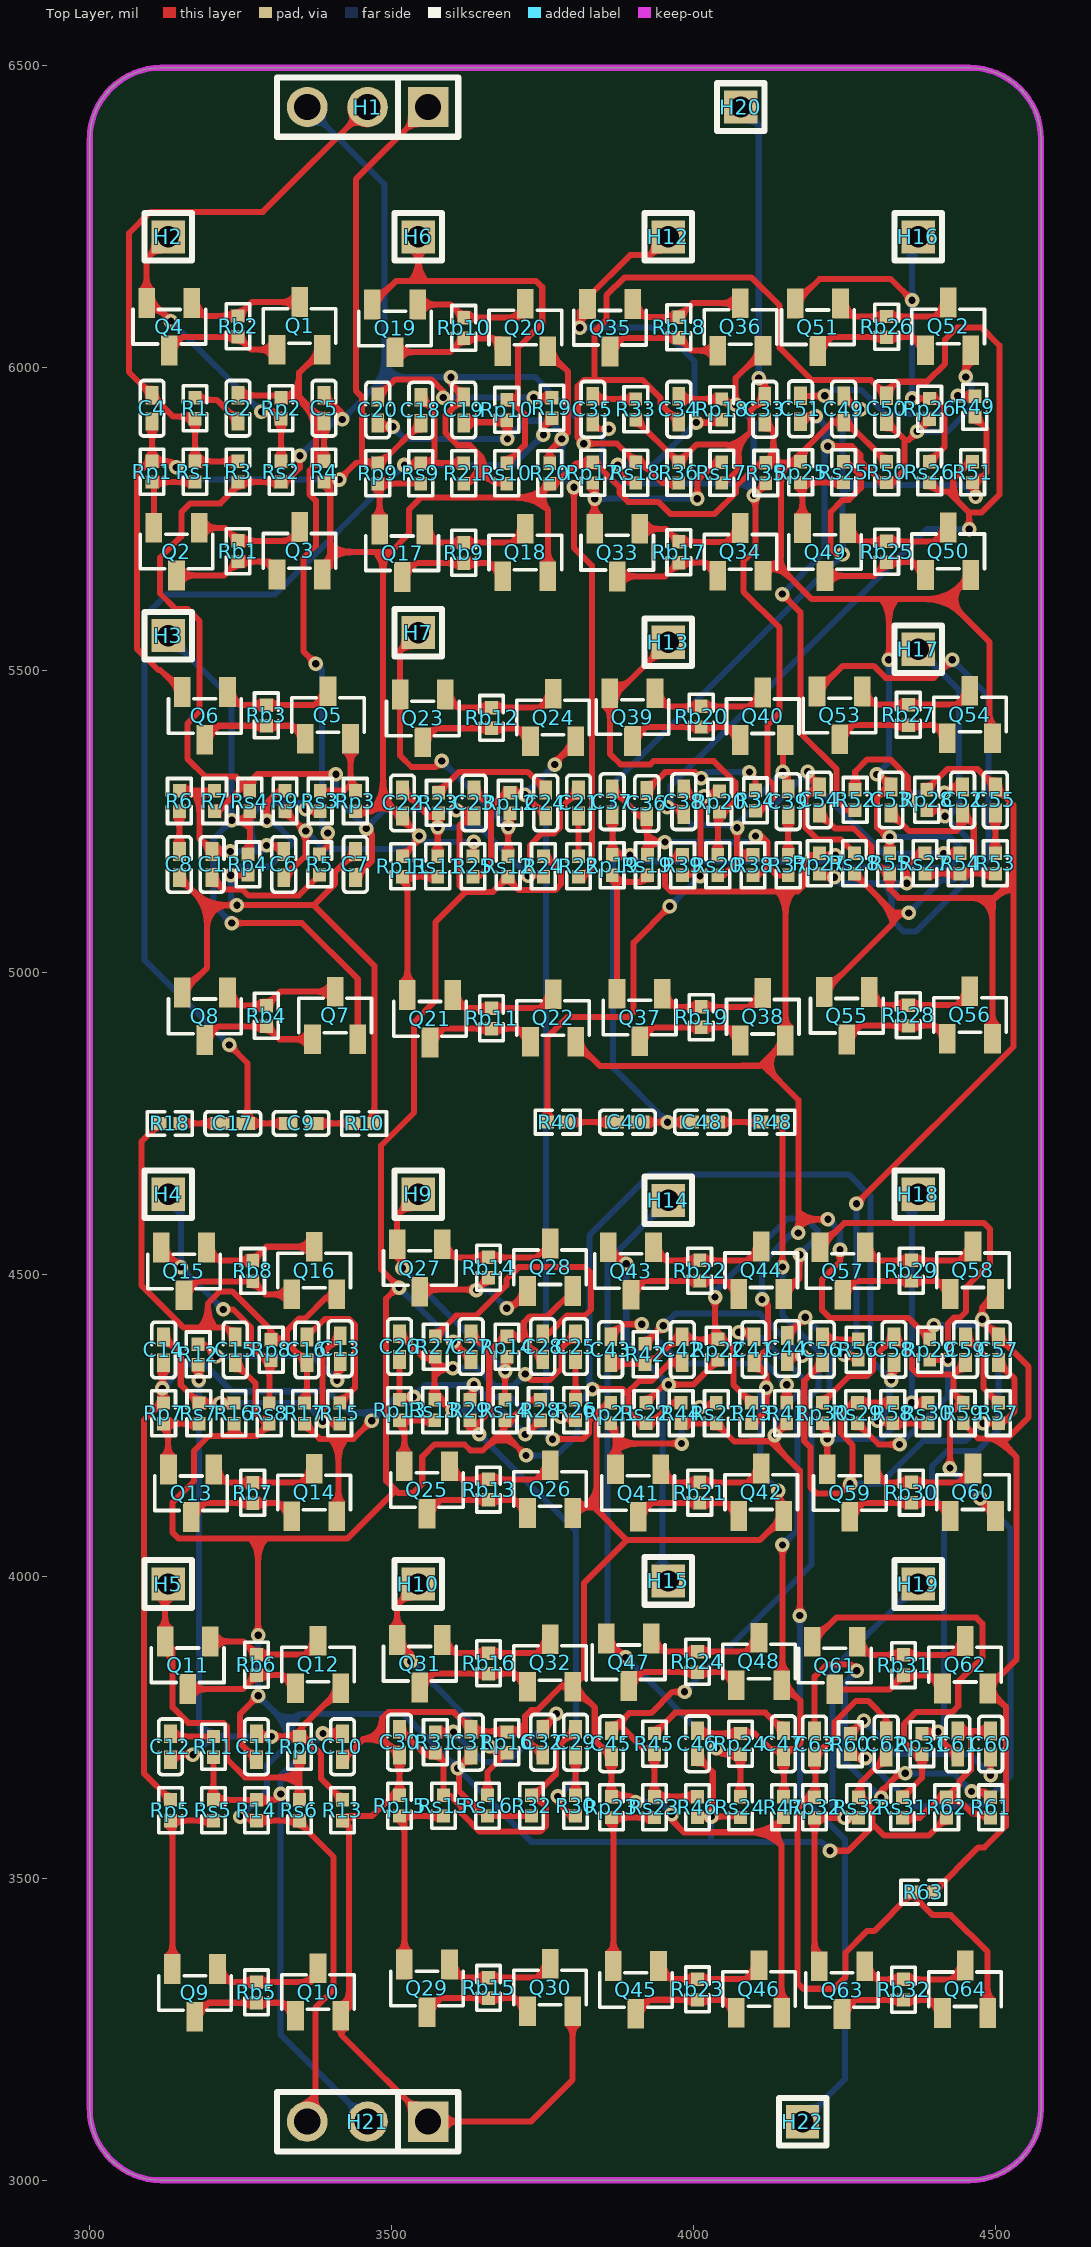
[diagram p0: Top Layer view]
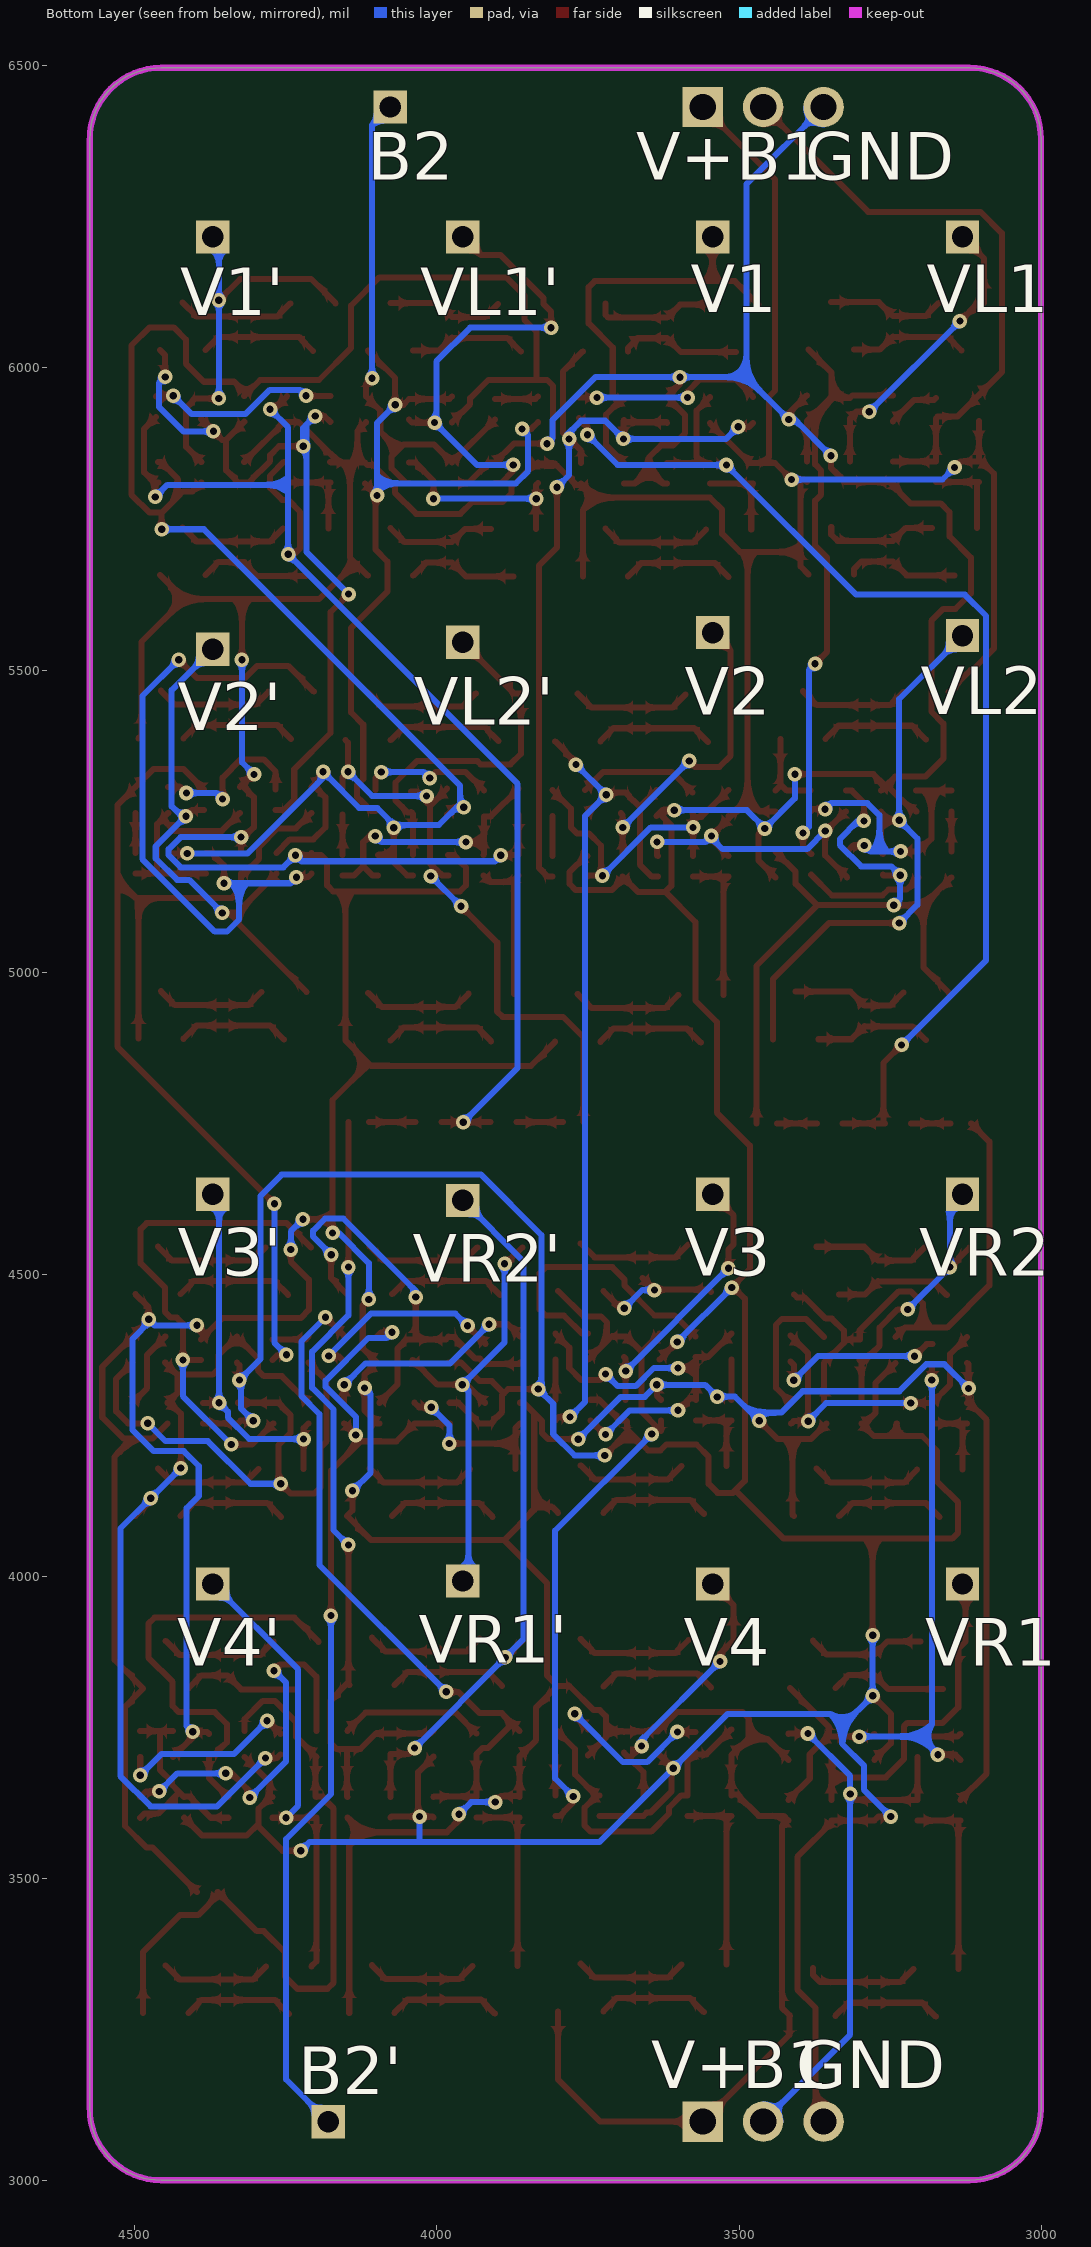
[diagram p1: Bottom Layer view, seen from below]
# Altium PCB MISC61260.pcbdoc (part 1 of 4)
Units mil, origin at the board's own origin, x right, y up, seen from the top; angles counter-clockwise.
Board outline 1574.8 x 3497.01 mil, 2 copper layers (Top Layer, Bottom Layer), stack 62.206 mil thick; 303 components, 159 nets, 654 pads, 177 vias.

## Layer stack, top to bottom
Top Solder Mask Layer: solder mask 0.394, Dk 3.3
Top Layer: signal copper 1.379
Dielectric1: surface 59.449, FR4, Dk 4.5
Bottom Layer: signal copper 1.378
Bottom Solder Mask Layer: solder mask 0.394, Dk 3.3

## Board outline
3118.11,6497.01 ccw(c3118.11,6378.9) 3000,6378.9 3000,3118.11 ccw(c3118.11,3118.11) 3118.11,3000 4456.69,3000 ccw(c4456.69,3118.11) 4574.8,3118.11 4574.8,6378.9 ccw(c4456.69,6378.9) 4456.69,6497.01 3118.11,6497.01

## Design rules (kind name [scope] priority, off if disabled: settings)
BoardOutlineClearance copperThickness2oz_1 [All] p2 off: genericclearance=7.99 ignorepadtopadclearanceinfootprint=FALSE except(0: Arc-SplitContinuation Track-SplitContinuation SMDPad-SplitContinuation THPad-SplitContinuation Via-SplitContinuation Fill-SplitContinuation Region-SplitContinuation Poly-SplitContinuation Text-SplitContinuation Hole-SplitContinuation; 5.98: Arc-CutoutEdge Track-CutoutEdge SMDPad-CutoutEdge THPad-CutoutEdge Via-CutoutEdge Text-CutoutEdge; 6.9: Hole-OutlineEdge Hole-CutoutEdge; 10: Poly-OutlineEdge Poly-CutoutEdge; 11.81: Arc-OutlineEdge Track-OutlineEdge SMDPad-OutlineEdge THPad-OutlineEdge Via-OutlineEdge Fill-OutlineEdge Region-OutlineEdge Text-OutlineEdge Fill-CutoutEdge Region-CutoutEdge)
BoardOutlineClearance Plane_innerPlane_1 [All] p4 off: genericclearance=4.02 ignorepadtopadclearanceinfootprint=FALSE except(0: Arc-SplitContinuation Track-SplitContinuation SMDPad-SplitContinuation THPad-SplitContinuation Via-SplitContinuation Fill-SplitContinuation Region-SplitContinuation Poly-SplitContinuation Text-SplitContinuation Hole-SplitContinuation; 5.98: Arc-CutoutEdge Track-CutoutEdge SMDPad-CutoutEdge THPad-CutoutEdge Via-CutoutEdge Text-CutoutEdge; 6.9: Hole-OutlineEdge Hole-CutoutEdge; 10: Poly-OutlineEdge Poly-CutoutEdge; 11.81: Arc-OutlineEdge Track-OutlineEdge SMDPad-OutlineEdge THPad-OutlineEdge Via-OutlineEdge Fill-OutlineEdge Region-OutlineEdge Text-OutlineEdge Fill-CutoutEdge Region-CutoutEdge)
BoardOutlineClearance Copper_copperRegion_1 [All] p6 off: genericclearance=4.02 ignorepadtopadclearanceinfootprint=FALSE except(0: Arc-SplitContinuation Track-SplitContinuation SMDPad-SplitContinuation THPad-SplitContinuation Via-SplitContinuation Fill-SplitContinuation Region-SplitContinuation Poly-SplitContinuation Text-SplitContinuation Hole-SplitContinuation; 5.98: Arc-CutoutEdge Track-CutoutEdge SMDPad-CutoutEdge THPad-CutoutEdge Via-CutoutEdge Text-CutoutEdge; 6.9: Hole-OutlineEdge Hole-CutoutEdge; 10: Poly-OutlineEdge Poly-CutoutEdge; 11.81: Arc-OutlineEdge Track-OutlineEdge SMDPad-OutlineEdge THPad-OutlineEdge Via-OutlineEdge Fill-OutlineEdge Region-OutlineEdge Text-OutlineEdge Fill-CutoutEdge Region-CutoutEdge)
BoardOutlineClearance copperThickness1oz_1 [All] p8: genericclearance=4.02 ignorepadtopadclearanceinfootprint=FALSE except(0: Arc-SplitContinuation Track-SplitContinuation SMDPad-SplitContinuation THPad-SplitContinuation Via-SplitContinuation Fill-SplitContinuation Region-SplitContinuation Poly-SplitContinuation Text-SplitContinuation Hole-SplitContinuation; 5.98: Arc-CutoutEdge Track-CutoutEdge SMDPad-CutoutEdge THPad-CutoutEdge Via-CutoutEdge Text-CutoutEdge; 6.9: Hole-OutlineEdge Hole-CutoutEdge; 10: Poly-OutlineEdge Poly-CutoutEdge; 11.81: Arc-OutlineEdge Track-OutlineEdge SMDPad-OutlineEdge THPad-OutlineEdge Via-OutlineEdge Fill-OutlineEdge Region-OutlineEdge Text-OutlineEdge Fill-CutoutEdge Region-CutoutEdge)
Clearance copperThickness2oz [All] p1 off: gap=7.99 ignorepadtopadclearanceinfootprint=FALSE except(5.98: SMDPad-Track SMDPad-SMDPad THPad-Track SMDPad-THPad THPad-THPad Track-Via SMDPad-Via THPad-Via Via-Via Fill-SMDPad Region-SMDPad Fill-THPad Region-THPad Fill-Via Region-Via Fill-Fill Fill-Region Region-Region Arc-Track Arc-SMDPad Arc-THPad Arc-Via Fill-Arc Region-Arc Arc-Arc Text-Track SMDPad-Text Text-THPad Text-Via Fill-Text Region-Text Arc-Text Text-Text; 6.9: Hole-Track Hole-SMDPad Hole-THPad Hole-Via Fill-Hole Region-Hole Hole-Arc Hole-Text; 10: Poly-Track Poly-SMDPad Poly-THPad Poly-Via Poly-Fill Poly-Region Poly-Poly Poly-Arc Poly-Text Poly-Hole; 11.81: Fill-Track Region-Track)
Clearance Plane_innerPlane [All] p3 off: gap=4.02 ignorepadtopadclearanceinfootprint=FALSE except(5.98: SMDPad-Track SMDPad-SMDPad THPad-Track SMDPad-THPad THPad-THPad Track-Via SMDPad-Via THPad-Via Via-Via Fill-SMDPad Region-SMDPad Fill-THPad Region-THPad Fill-Via Region-Via Fill-Fill Fill-Region Region-Region Arc-Track Arc-SMDPad Arc-THPad Arc-Via Fill-Arc Region-Arc Arc-Arc Text-Track SMDPad-Text Text-THPad Text-Via Fill-Text Region-Text Arc-Text Text-Text; 6.9: Hole-Track Hole-SMDPad Hole-THPad Hole-Via Fill-Hole Region-Hole Hole-Arc Hole-Text; 10: Poly-Track Poly-SMDPad Poly-THPad Poly-Via Poly-Fill Poly-Region Poly-Poly Poly-Arc Poly-Text Poly-Hole; 11.81: Fill-Track Region-Track)
Clearance Copper_copperRegion [All] p5 off: gap=4.02 ignorepadtopadclearanceinfootprint=FALSE except(5.98: SMDPad-Track SMDPad-SMDPad THPad-Track SMDPad-THPad THPad-THPad Track-Via SMDPad-Via THPad-Via Via-Via Fill-SMDPad Region-SMDPad Fill-THPad Region-THPad Fill-Via Region-Via Fill-Fill Fill-Region Region-Region Arc-Track Arc-SMDPad Arc-THPad Arc-Via Fill-Arc Region-Arc Arc-Arc Text-Track SMDPad-Text Text-THPad Text-Via Fill-Text Region-Text Arc-Text Text-Text; 6.9: Hole-Track Hole-SMDPad Hole-THPad Hole-Via Fill-Hole Region-Hole Hole-Arc Hole-Text; 10: Poly-Track Poly-SMDPad Poly-THPad Poly-Via Poly-Fill Poly-Region Poly-Poly Poly-Arc Poly-Text Poly-Hole; 11.81: Fill-Track Region-Track)
Clearance copperThickness1oz [All] p7: gap=4.02 ignorepadtopadclearanceinfootprint=FALSE except(5.98: SMDPad-Track SMDPad-SMDPad THPad-Track SMDPad-THPad THPad-THPad Track-Via SMDPad-Via THPad-Via Via-Via Fill-SMDPad Region-SMDPad Fill-THPad Region-THPad Fill-Via Region-Via Fill-Fill Fill-Region Region-Region Arc-Track Arc-SMDPad Arc-THPad Arc-Via Fill-Arc Region-Arc Arc-Arc Text-Track SMDPad-Text Text-THPad Text-Via Fill-Text Region-Text Arc-Text Text-Text; 6.9: Hole-Track Hole-SMDPad Hole-THPad Hole-Via Fill-Hole Region-Hole Hole-Arc Hole-Text; 10: Poly-Track Poly-SMDPad Poly-THPad Poly-Via Poly-Fill Poly-Region Poly-Poly Poly-Arc Poly-Text Poly-Hole; 11.81: Fill-Track Region-Track)
DiffPairsRouting differentialPair [All] p1: maxlimit=6 minlimit=6 mostfreqgap=6 toplayer_minwidth=5 toplayer_prefwidth=10 toplayer_maxwidth=100 toplayer_mingap=6 toplayer_prefgap=6 toplayer_maxgap=6 bottomlayer_minwidth=5 bottomlayer_prefwidth=10 bottomlayer_maxwidth=100 bottomlayer_mingap=6 bottomlayer_prefgap=6 bottomlayer_maxgap=6 maxuncoupledlength=10
HoleToHoleClearance otherClearance [All] p1: gap=11.81 allowstackedmicrovias=TRUE
Length netLength [All] p1: minlimit=0 maxlimit=0
PasteMaskExpansion pasteMaskExpansion [All] p1: expansion=0
PlaneConnect innerPlane [All] p1: planeconnectstyle=Relief reliefexpansion=20 reliefentries=4 reliefconductorwidth=10 reliefairgap=10
PolygonConnect copperRegion [All] p1: connectstyle=Relief reliefconductorwidth=10 reliefentries=4 polygonreliefangle="90 Angle" airgapwidth=10 via.connectstyle=Relief via.reliefconductorwidth=10 via.reliefentries=4 via.polygonreliefangle="90 Angle" via.airgapwidth=10
RoutingVias viaSize [All] p1: holewidth=12.01 width=24.02 viastyle="Through Hole" minholewidth=11.81 minwidth=19.68 maxholewidth=248.03 maxwidth=393.7
SolderMaskExpansion solderMaskExpansion [IsVia] p1: expansion=-1000 istentingtop=TRUE
SolderMaskExpansion solderMaskExpansion [All] p2: expansion=2 istentingtop=FALSE
Width copperThickness2oz_2 [All] p1 off: maxlimit=100 minlimit=8 preferedwidth=10
Width copperThickness1oz_2 [All] p2: maxlimit=100 minlimit=5 preferedwidth=10

## Components (designator, comment, footprint, x,y, rotation, side; value= is the part's Value field where it differs from the comment)
C1 "0.1uF" C0402 3202.63,5178.18 r270 top
C2 "0.1uF" C0402 3245.47,5933.34 r270 top
C4 "0.1uF" C0402 3103.12,5933.34 r90 top
C5 "0.1uF" C0402 3387.83,5933.34 r90 top
C6 "0.1uF" C0402 3321.19,5178.18 r90 top
C7 "0.1uF" C0402 3439.75,5178.18 r270 top
C8 "0.1uF" C0402 3148.35,5178.18 r90 top
C9 "0.02uF" C0402 3349.88,4749.42 r0 top
C10 "0.1uF" C0402 3418.31,3717.49 r90 top
C11 "0.1uF" C0402 3275.95,3717.49 r270 top
C12 "0.1uF" C0402 3133.6,3717.49 r90 top
C13 "0.1uF" C0402 3414.58,4376.59 r270 top
C14 "0.1uF" C0402 3122.33,4374.57 r90 top
C15 "0.1uF" C0402 3240.89,4374.57 r270 top
C16 "0.1uF" C0402 3359.45,4374.57 r90 top
C17 "0.02uF" C0402 3236.81,4749.42 r180 top
C18 "0.1uF" C0402 3548.14,5930.15 r90 top
C19 "0.1uF" C0402 3619.09,5930.63 r90 top
C20 "0.1uF" C0402 3476.74,5930.63 r90 top
C21 "0.1uF" C0402 3809.15,5279.99 r270 top
C22 "0.1uF" C0402 3517.75,5279.99 r90 top
C23 "0.1uF" C0402 3636.31,5279.99 r270 top
C24 "0.1uF" C0402 3754.87,5279.99 r90 top
C25 "0.1uF" C0402 3804.15,4379.99 r270 top
C26 "0.1uF" C0402 3512.75,4379.99 r90 top
C27 "0.1uF" C0402 3631.31,4379.99 r270 top
C28 "0.1uF" C0402 3749.87,4379.99 r90 top
C29 "0.1uF" C0402 3804.15,3724.99 r270 top
C30 "0.1uF" C0402 3512.75,3724.99 r90 top
C31 "0.1uF" C0402 3631.31,3724.99 r270 top
C32 "0.1uF" C0402 3749.87,3724.99 r90 top
C33 "0.1uF" C0402 4117.46,5931.65 r90 top
C34 "0.1uF" C0402 3975.11,5931.65 r270 top
C35 "0.1uF" C0402 3832.75,5931.65 r90 top
C36 "0.1uF" C0402 3922.08,5279.09 r90 top
C37 "0.1uF" C0402 3864.83,5282.07 r90 top
C38 "0.1uF" C0402 3983.39,5282.07 r270 top
C39 "0.1uF" C0402 4156.23,5282.07 r270 top
C40 "0.02uF" C0402 3889.96,4751.59 r180 top
C41 "0.1uF" C0402 4099.45,4374.99 r90 top
C42 "0.1uF" C0402 3980.89,4374.99 r270 top
C43 "0.1uF" C0402 3862.33,4374.99 r90 top
C44 "0.1uF" C0402 4154.58,4377.01 r270 top
C45 "0.1uF" C0402 3863.6,3722.49 r90 top
C46 "0.1uF" C0402 4005.95,3722.49 r270 top
C47 "0.1uF" C0402 4148.31,3722.49 r90 top
C48 "0.02uF" C0402 4014.19,4751.59 r0 top
C49 "0.1uF" C0402 4248.14,5932.01 r90 top
C50 "0.1uF" C0402 4319.09,5932.49 r90 top
C51 "0.1uF" C0402 4176.74,5932.49 r90 top
C52 "0.1uF" C0402 4444.87,5284.99 r90 top
C53 "0.1uF" C0402 4326.31,5284.99 r270 top
C54 "0.1uF" C0402 4207.75,5284.99 r90 top
C55 "0.1uF" C0402 4499.15,5284.99 r270 top
C56 "0.1uF" C0402 4212.75,4374.99 r90 top
C57 "0.1uF" C0402 4504.15,4374.99 r270 top
C58 "0.1uF" C0402 4331.31,4374.99 r270 top
C59 "0.1uF" C0402 4449.87,4374.99 r90 top
C60 "0.1uF" C0402 4491.23,3722.07 r270 top
C61 "0.1uF" C0402 4436.95,3722.07 r90 top
C62 "0.1uF" C0402 4318.39,3722.07 r270 top
C63 "0.1uF" C0402 4199.83,3722.07 r90 top
H1 "" HDR-TH_3P-P2.54-V-M 3460,6432.01 r180 top
H2 "" HDR-TH_1P-V-M_XKB_X4611WV-01I-C28D40 3130,6217.01 r0 top
H3 "" HDR-TH_1P-V-M_XKB_X4611WV-01I-C28D40 3130,5557.01 r0 top
H4 "" HDR-TH_1P-V-M_XKB_X4611WV-01I-C28D40 3130,4632.01 r0 top
H5 "" HDR-TH_1P-V-M_XKB_X4611WV-01I-C28D40 3130,3987.01 r0 top
H6 "" HDR-TH_1P-V-M_XKB_X4611WV-01I-C28D40 3543.75,6217.01 r0 top
H7 "" HDR-TH_1P-V-M_XKB_X4611WV-01I-C28D40 3543.75,5562.01 r0 top
H9 "" HDR-TH_1P-V-M_XKB_X4611WV-01I-C28D40 3543.75,4632.01 r0 top
H10 "" HDR-TH_1P-V-M_XKB_X4611WV-01I-C28D40 3543.75,3987.01 r0 top
H12 "" HDR-TH_1P-V-M_XKB_X4611WV-01I-C28D40 3957.5,6217.01 r0 top
H13 "" HDR-TH_1P-V-M_XKB_X4611WV-01I-C28D40 3957.5,5546.15 r0 top
H14 "" HDR-TH_1P-V-M_XKB_X4611WV-01I-C28D40 3957.5,4622.01 r0 top
H15 "" HDR-TH_1P-V-M_XKB_X4611WV-01I-C28D40 3957.5,3992.01 r0 top
H16 "" HDR-TH_1P-V-M_XKB_X4611WV-01I-C28D40 4371.25,6217.01 r0 top
H17 "" HDR-TH_1P-V-M_XKB_X4611WV-01I-C28D40 4371.25,5534.57 r0 top
H18 "" HDR-TH_1P-V-M_XKB_X4611WV-01I-C28D40 4371.25,4632.01 r0 top
H19 "" HDR-TH_1P-V-M_XKB_X4611WV-01I-C28D40 4371.25,3987.01 r0 top
H20 "" HDR-TH_1P-V-M_XKB_X4611WV-01I-C28D40 4077.5,6432.01 r0 top
H21 "" HDR-TH_3P-P2.54-V-M 3460,3097.01 r180 top
H22 "" HDR-TH_1P-V-M_XKB_X4611WV-01I-C28D40 4180,3097.01 r0 top
Q1 "MMBT3906" SOT-23-3_L2.9-W1.3-P1.90-LS2.4-BR 3347.37,6069.72 r270 top
Q2 "MMBT3904" SOT-23-3_L2.9-W1.3-P1.90-LS2.4-BR 3143.57,5696 r90 top
Q3 "MMBT3906" SOT-23-3_L2.9-W1.3-P1.90-LS2.4-BR 3347.37,5697.38 r270 top
Q4 "MMBT3904" SOT-23-3_L2.9-W1.3-P1.90-LS2.4-BR 3131.67,6068.34 r90 top
Q5 "MMBT3904" SOT-23-3_L2.9-W1.3-P1.90-LS2.4-BR 3394.29,5425.53 r270 top
Q6 "MMBT3906" SOT-23-3_L2.9-W1.3-P1.90-LS2.4-BR 3190.49,5424.15 r90 top
Q7 "MMBT3904" SOT-23-3_L2.9-W1.3-P1.90-LS2.4-BR 3406.2,4928.18 r270 top
Q8 "MMBT3906" SOT-23-3_L2.9-W1.3-P1.90-LS2.4-BR 3190.49,4926.8 r90 top
Q9 "MMBT3904" SOT-23-3_L2.9-W1.3-P1.90-LS2.4-BR 3174.06,3310.14 r90 top
Q10 "MMBT3906" SOT-23-3_L2.9-W1.3-P1.90-LS2.4-BR 3377.85,3311.52 r270 top
Q11 "MMBT3904" SOT-23-3_L2.9-W1.3-P1.90-LS2.4-BR 3162.15,3852.49 r90 top
Q12 "MMBT3906" SOT-23-3_L2.9-W1.3-P1.90-LS2.4-BR 3377.85,3853.87 r270 top
Q13 "MMBT3904" SOT-23-3_L2.9-W1.3-P1.90-LS2.4-BR 3167.79,4137.22 r90 top
Q14 "MMBT3906" SOT-23-3_L2.9-W1.3-P1.90-LS2.4-BR 3371.58,4138.6 r270 top
Q15 "MMBT3904" SOT-23-3_L2.9-W1.3-P1.90-LS2.4-BR 3155.88,4504.57 r90 top
Q16 "MMBT3906" SOT-23-3_L2.9-W1.3-P1.90-LS2.4-BR 3371.58,4505.95 r270 top
Q17 "MMBT3904" SOT-23-3_L2.9-W1.3-P1.90-LS2.4-BR 3517.19,5693.28 r90 top
Q18 "MMBT3906" SOT-23-3_L2.9-W1.3-P1.90-LS2.4-BR 3720.99,5694.66 r270 top
Q19 "MMBT3904" SOT-23-3_L2.9-W1.3-P1.90-LS2.4-BR 3505.29,6065.63 r90 top
Q20 "MMBT3906" SOT-23-3_L2.9-W1.3-P1.90-LS2.4-BR 3720.99,6067.01 r270 top
Q21 "MMBT3904" SOT-23-3_L2.9-W1.3-P1.90-LS2.4-BR 3563.21,4922.64 r90 top
Q22 "MMBT3906" SOT-23-3_L2.9-W1.3-P1.90-LS2.4-BR 3767.01,4924.02 r270 top
Q23 "MMBT3904" SOT-23-3_L2.9-W1.3-P1.90-LS2.4-BR 3551.3,5419.99 r90 top
Q24 "MMBT3906" SOT-23-3_L2.9-W1.3-P1.90-LS2.4-BR 3767.01,5421.37 r270 top
Q25 "MMBT3904" SOT-23-3_L2.9-W1.3-P1.90-LS2.4-BR 3558.21,4142.64 r90 top
Q26 "MMBT3906" SOT-23-3_L2.9-W1.3-P1.90-LS2.4-BR 3762.01,4144.02 r270 top
Q27 "MMBT3904" SOT-23-3_L2.9-W1.3-P1.90-LS2.4-BR 3546.3,4509.99 r90 top
Q28 "MMBT3906" SOT-23-3_L2.9-W1.3-P1.90-LS2.4-BR 3762.01,4511.37 r270 top
Q29 "MMBT3904" SOT-23-3_L2.9-W1.3-P1.90-LS2.4-BR 3558.21,3317.64 r90 top
Q30 "MMBT3906" SOT-23-3_L2.9-W1.3-P1.90-LS2.4-BR 3762.01,3319.02 r270 top
Q31 "MMBT3904" SOT-23-3_L2.9-W1.3-P1.90-LS2.4-BR 3546.3,3854.99 r90 top
Q32 "MMBT3906" SOT-23-3_L2.9-W1.3-P1.90-LS2.4-BR 3762.01,3856.37 r270 top
Q33 "MMBT3904" SOT-23-3_L2.9-W1.3-P1.90-LS2.4-BR 3873.21,5694.3 r90 top
Q34 "MMBT3906" SOT-23-3_L2.9-W1.3-P1.90-LS2.4-BR 4077.01,5695.68 r270 top
Q35 "MMBT3904" SOT-23-3_L2.9-W1.3-P1.90-LS2.4-BR 3861.3,6066.65 r90 top
Q36 "MMBT3906" SOT-23-3_L2.9-W1.3-P1.90-LS2.4-BR 4077.01,6068.03 r270 top
Q37 "MMBT3904" SOT-23-3_L2.9-W1.3-P1.90-LS2.4-BR 3910.29,4924.72 r90 top
Q38 "MMBT3906" SOT-23-3_L2.9-W1.3-P1.90-LS2.4-BR 4114.08,4926.1 r270 top
Q39 "MMBT3904" SOT-23-3_L2.9-W1.3-P1.90-LS2.4-BR 3898.38,5422.07 r90 top
Q40 "MMBT3906" SOT-23-3_L2.9-W1.3-P1.90-LS2.4-BR 4114.08,5423.45 r270 top
Q41 "MMBT3904" SOT-23-3_L2.9-W1.3-P1.90-LS2.4-BR 3907.79,4137.64 r90 top
Q42 "MMBT3906" SOT-23-3_L2.9-W1.3-P1.90-LS2.4-BR 4111.58,4139.02 r270 top
Q43 "MMBT3904" SOT-23-3_L2.9-W1.3-P1.90-LS2.4-BR 3895.88,4504.99 r90 top
Q44 "MMBT3906" SOT-23-3_L2.9-W1.3-P1.90-LS2.4-BR 4111.58,4506.37 r270 top
Q45 "MMBT3904" SOT-23-3_L2.9-W1.3-P1.90-LS2.4-BR 3904.06,3315.14 r90 top
Q46 "MMBT3906" SOT-23-3_L2.9-W1.3-P1.90-LS2.4-BR 4107.85,3316.52 r270 top
Q47 "MMBT3904" SOT-23-3_L2.9-W1.3-P1.90-LS2.4-BR 3892.15,3857.49 r90 top
Q48 "MMBT3906" SOT-23-3_L2.9-W1.3-P1.90-LS2.4-BR 4107.85,3858.87 r270 top
Q49 "MMBT3904" SOT-23-3_L2.9-W1.3-P1.90-LS2.4-BR 4217.19,5695.14 r90 top
Q50 "MMBT3906" SOT-23-3_L2.9-W1.3-P1.90-LS2.4-BR 4420.99,5696.52 r270 top
Q51 "MMBT3904" SOT-23-3_L2.9-W1.3-P1.90-LS2.4-BR 4205.29,6067.49 r90 top
Q52 "MMBT3906" SOT-23-3_L2.9-W1.3-P1.90-LS2.4-BR 4420.99,6068.87 r270 top
Q53 "MMBT3904" SOT-23-3_L2.9-W1.3-P1.90-LS2.4-BR 4241.3,5424.99 r90 top
Q54 "MMBT3906" SOT-23-3_L2.9-W1.3-P1.90-LS2.4-BR 4457.01,5426.37 r270 top
Q55 "MMBT3904" SOT-23-3_L2.9-W1.3-P1.90-LS2.4-BR 4253.21,4927.64 r90 top
Q56 "MMBT3906" SOT-23-3_L2.9-W1.3-P1.90-LS2.4-BR 4457.01,4929.02 r270 top
Q57 "MMBT3904" SOT-23-3_L2.9-W1.3-P1.90-LS2.4-BR 4246.3,4504.99 r90 top
Q58 "MMBT3906" SOT-23-3_L2.9-W1.3-P1.90-LS2.4-BR 4462.01,4506.37 r270 top
Q59 "MMBT3904" SOT-23-3_L2.9-W1.3-P1.90-LS2.4-BR 4258.21,4137.64 r90 top
Q60 "MMBT3906" SOT-23-3_L2.9-W1.3-P1.90-LS2.4-BR 4462.01,4139.02 r270 top
Q61 "MMBT3904" SOT-23-3_L2.9-W1.3-P1.90-LS2.4-BR 4233.38,3852.07 r90 top
Q62 "MMBT3906" SOT-23-3_L2.9-W1.3-P1.90-LS2.4-BR 4449.08,3853.45 r270 top
Q63 "MMBT3904" SOT-23-3_L2.9-W1.3-P1.90-LS2.4-BR 4245.29,3314.72 r90 top
Q64 "MMBT3906" SOT-23-3_L2.9-W1.3-P1.90-LS2.4-BR 4449.08,3316.1 r270 top
R1 "1" R0402 3174.29,5933.34 r270 top
R3 "2.2K" R0402 3245.47,5828.34 r270 top
R4 "2.2K" R0402 3387.83,5828.34 r90 top
R5 "1" R0402 3380.47,5178.18 r90 top
R6 "1" R0402 3148.35,5283.18 r90 top
R7 "2.2K" R0402 3206.63,5283.18 r270 top
R9 "2.2K" R0402 3323.19,5283.18 r90 top
R10 "1" R0402 3454.1,4749.42 r0 top
R11 "1" R0402 3204.78,3717.49 r270 top
R12 "1" R0402 3179.35,4367.07 r270 top
R13 "2.2K" R0402 3418.31,3612.49 r90 top
R14 "2.2K" R0402 3275.95,3612.49 r270 top
R15 "1" R0402 3413.73,4269.57 r270 top
R16 "2.2K" R0402 3238.89,4269.57 r270 top
R17 "2.2K" R0402 3355.45,4269.57 r90 top
R18 "1" R0402 3132.59,4749.42 r180 top
R19 "1" R0402 3765.17,5934.05 r270 top
R20 "2.2K" R0402 3761.45,5825.63 r90 top
R21 "2.55K" R0402 3619.09,5825.63 r270 top
R22 "1" R0402 3809.15,5174.99 r270 top
R23 "1" R0402 3577.03,5279.99 r270 top
R24 "2.2K" R0402 3750.87,5174.99 r90 top
R25 "2.2K" R0402 3634.31,5174.99 r270 top
R26 "1" R0402 3804.15,4274.99 r270 top
R27 "1" R0402 3572.03,4379.99 r270 top
R28 "2.2K" R0402 3745.87,4274.99 r90 top
R29 "2.2K" R0402 3629.31,4274.99 r270 top
R30 "1" R0402 3804.15,3619.99 r270 top
R31 "1" R0402 3572.03,3724.99 r270 top
R32 "2.2K" R0402 3731.3,3619.99 r270 top
R33 "1" R0402 3903.93,5931.65 r270 top
R34 "1" R0402 4102.08,5284.09 r270 top
R35 "2.2K" R0402 4119.15,5826.16 r270 top
R36 "2.2K" R0402 3975.11,5826.65 r270 top
R37 "1" R0402 4156.23,5177.07 r270 top
R38 "2.2K" R0402 4097.95,5177.07 r90 top
R39 "2.2K" R0402 3981.39,5177.07 r270 top
R40 "1" R0402 3774.58,4751.59 r180 top
R41 "1" R0402 4153.73,4269.99 r270 top
R42 "1" R0402 3919.35,4367.49 r270 top
R43 "2.2K" R0402 4095.45,4269.99 r90 top
R44 "2.2K" R0402 3978.89,4269.99 r90 top
R45 "1" R0402 3934.78,3722.49 r270 top
R46 "2.2K" R0402 4005.95,3617.49 r270 top
R47 "2.2K" R0402 4148.31,3617.49 r90 top
R48 "1" R0402 4129.58,4751.59 r0 top
R49 "1" R0402 4465.17,5935.91 r270 top
R50 "2.2K" R0402 4319.09,5827.49 r270 top
R51 "2.55K" R0402 4461.45,5827.49 r90 top
R52 "1" R0402 4267.03,5284.99 r270 top
R53 "1" R0402 4499.15,5179.99 r270 top
R54 "2.2K" R0402 4440.87,5179.99 r90 top
R55 "2.2K" R0402 4324.31,5179.99 r270 top
R56 "1" R0402 4272.03,4374.99 r270 top
R57 "1" R0402 4504.15,4269.99 r270 top
R58 "2.2K" R0402 4329.31,4269.99 r270 top
R59 "2.2K" R0402 4445.87,4269.99 r90 top
R60 "1" R0402 4259.11,3722.07 r270 top
R61 "1" R0402 4491.23,3617.07 r270 top
R62 "2.2K" R0402 4418.38,3617.07 r270 top
R63 "2.2K" R0402 4380,3477.01 r180 top
Rb1 "1K" R0402 3245.47,5696.69 r270 top
Rb2 "1K" R0402 3245.47,6069.03 r270 top
Rb3 "1K" R0402 3292.39,5424.84 r90 top
Rb4 "1K" R0402 3292.39,4927.49 r90 top
Rb5 "1K" R0402 3275.95,3310.83 r270 top
Rb6 "1K" R0402 3275.95,3853.18 r270 top
Rb7 "1K" R0402 3269.68,4137.91 r270 top
Rb8 "1K" R0402 3269.68,4505.26 r270 top
Rb9 "1K" R0402 3619.09,5693.97 r270 top
Rb10 "1K" R0402 3619.09,6066.32 r270 top
Rb11 "1K" R0402 3665.11,4923.33 r270 top
Rb12 "1K" R0402 3665.11,5420.68 r270 top
Rb13 "1K" R0402 3660.11,4143.33 r270 top
Rb14 "1K" R0402 3660.11,4510.68 r270 top
Rb15 "1K" R0402 3660.11,3318.33 r270 top
Rb16 "1K" R0402 3660.11,3855.68 r270 top
Rb17 "1K" R0402 3975.11,5694.99 r270 top
Rb18 "1K" R0402 3975.11,6067.34 r270 top
Rb19 "1K" R0402 4012.18,4925.41 r270 top
Rb20 "1K" R0402 4012.18,5422.76 r270 top
Rb21 "1K" R0402 4009.68,4138.33 r270 top
Rb22 "1K" R0402 4009.68,4505.68 r270 top
Rb23 "1K" R0402 4005.95,3315.83 r270 top
Rb24 "1K" R0402 4005.95,3858.18 r270 top
Rb25 "1K" R0402 4319.09,5695.83 r270 top
Rb26 "1K" R0402 4319.09,6068.18 r270 top
Rb27 "1K" R0402 4355.11,5425.68 r270 top
Rb28 "1K" R0402 4355.11,4928.33 r270 top
Rb29 "1K" R0402 4360.11,4505.68 r270 top
Rb30 "1K" R0402 4360.11,4138.33 r270 top
Rb31 "1K" R0402 4347.18,3852.76 r270 top
Rb32 "1K" R0402 4347.18,3315.41 r270 top
Rp1 "200K" R0402 3103.12,5828.34 r270 top
Rp2 "200K" R0402 3316.65,5933.34 r270 top
Rp3 "200K" R0402 3439.75,5283.18 r90 top
Rp4 "200K" R0402 3261.91,5178.18 r90 top
Rp5 "200K" R0402 3133.6,3612.49 r270 top
Rp6 "200K" R0402 3347.13,3717.49 r270 top
Rp7 "200K" R0402 3122.33,4269.57 r270 top
Rp8 "200K" R0402 3300.17,4374.57 r270 top
Rp9 "200K" R0402 3476.74,5825.63 r270 top
Rp10 "200K" R0402 3690.27,5930.63 r90 top
Rp11 "200K" R0402 3517.75,5174.99 r270 top
Rp12 "200K" R0402 3695.59,5279.99 r270 top
Rp13 "200K" R0402 3512.75,4274.99 r270 top
Rp14 "200K" R0402 3690.59,4379.99 r270 top
Rp15 "200K" R0402 3512.75,3619.99 r270 top
Rp16 "200K" R0402 3690.59,3724.99 r270 top
Rp17 "200K" R0402 3832.75,5826.65 r270 top
Rp18 "200K" R0402 4046.29,5931.65 r270 top
Rp19 "200K" R0402 3864.83,5177.07 r270 top
Rp20 "200K" R0402 4042.67,5282.07 r270 top
Rp21 "200K" R0402 3862.33,4269.99 r270 top
Rp22 "200K" R0402 4040.17,4374.99 r270 top
Rp23 "200K" R0402 3863.6,3617.49 r270 top
Rp24 "200K" R0402 4077.13,3722.49 r270 top
Rp25 "200K" R0402 4176.74,5827.49 r270 top
Rp26 "200K" R0402 4390.27,5932.49 r90 top
Rp27 "200K" R0402 4207.75,5179.99 r270 top
Rp28 "200K" R0402 4385.59,5284.99 r270 top
Rp29 "200K" R0402 4390.59,4374.99 r270 top
Rp30 "200K" R0402 4212.75,4269.99 r270 top
Rp31 "200K" R0402 4377.67,3722.07 r270 top
Rp32 "200K" R0402 4199.83,3617.07 r270 top
Rs1 "200" R0402 3174.29,5828.34 r90 top
Rs2 "200" R0402 3316.65,5828.34 r270 top
Rs3 "200" R0402 3381.47,5283.18 r270 top
Rs4 "200" R0402 3264.91,5283.18 r90 top
Rs5 "200" R0402 3204.78,3612.49 r90 top
Rs6 "200" R0402 3347.13,3612.49 r270 top
Rs7 "200" R0402 3180.61,4269.57 r90 top
Rs8 "200" R0402 3297.17,4269.57 r270 top
Rs9 "200" R0402 3547.91,5825.63 r90 top
Rs10 "200" R0402 3690.27,5825.63 r270 top
Rs11 "200" R0402 3576.03,5174.99 r90 top
Rs12 "200" R0402 3692.59,5174.99 r270 top
Rs13 "200" R0402 3571.03,4274.99 r90 top
Rs14 "200" R0402 3687.59,4274.99 r270 top
Rs15 "200" R0402 3585.6,3619.99 r90 top
Rs16 "200" R0402 3658.45,3619.99 r270 top
Rs17 "200" R0402 4046.29,5826.65 r270 top
Rs18 "200" R0402 3903.93,5826.65 r90 top
Rs19 "200" R0402 3923.11,5177.07 r90 top
Rs20 "200" R0402 4039.67,5177.07 r270 top
Rs21 "200" R0402 4037.17,4269.99 r270 top
Rs22 "200" R0402 3920.61,4269.99 r270 top
Rs23 "200" R0402 3934.78,3617.49 r90 top
Rs24 "200" R0402 4077.13,3617.49 r270 top
Rs25 "200" R0402 4247.91,5827.49 r90 top
Rs26 "200" R0402 4390.27,5827.49 r270 top
Rs27 "200" R0402 4382.59,5179.99 r270 top
Rs28 "200" R0402 4266.03,5179.99 r90 top
Rs29 "200" R0402 4271.03,4269.99 r90 top
Rs30 "200" R0402 4387.59,4269.99 r270 top
Rs31 "200" R0402 4345.53,3617.07 r270 top
Rs32 "200" R0402 4272.68,3617.07 r90 top

## Footprints (in the part's own frame and the unit in brackets; to place one, negate y for a bottom-side part, rotate by r counter-clockwise, add the part's x,y. Pads: shape width x height; smd on the part's side, far side on the other; paste and mask are expansions set on the pad)
C0402 [mm]
  rect 0.79x0.54 smd paste-100 mask+0.051: 1(-0.545,0) 2(0.545,0)
  silkscreen extent -1.17,-0.5 1.17,0.5
HDR-TH_1P-V-M_XKB_X4611WV-01I-C28D40 [mm]
  rect 1.4x1.4 hole 0.9: 1(0,0)
  silkscreen extent -1,-1 1,1
HDR-TH_3P-P2.54-V-M [mm]
  rect 1.7x1.7 hole 1.1: 1(-2.54,0)
  round 1.7 hole 1.1: 2(0,0) 3(2.54,0)
  silkscreen extent -3.81,-1.25 3.81,1.25
R0402 [mm]
  rect 0.566x0.54 smd paste-100 mask+0.051: 1(-0.433,0) 2(0.433,0)
  silkscreen extent -0.94,-0.5 0.94,0.5
SOT-23-3_L2.9-W1.3-P1.90-LS2.4-BR [mm]
  rect 1.25x0.7 smd: 1(1,-0.95) 2(1,0.95) 3(-1,0)
  silkscreen extent -0.73,-1.53 0.73,1.53

## Via types
v1: diameter 24.02, hole 12, Top Layer to Bottom Layer, 177 vias